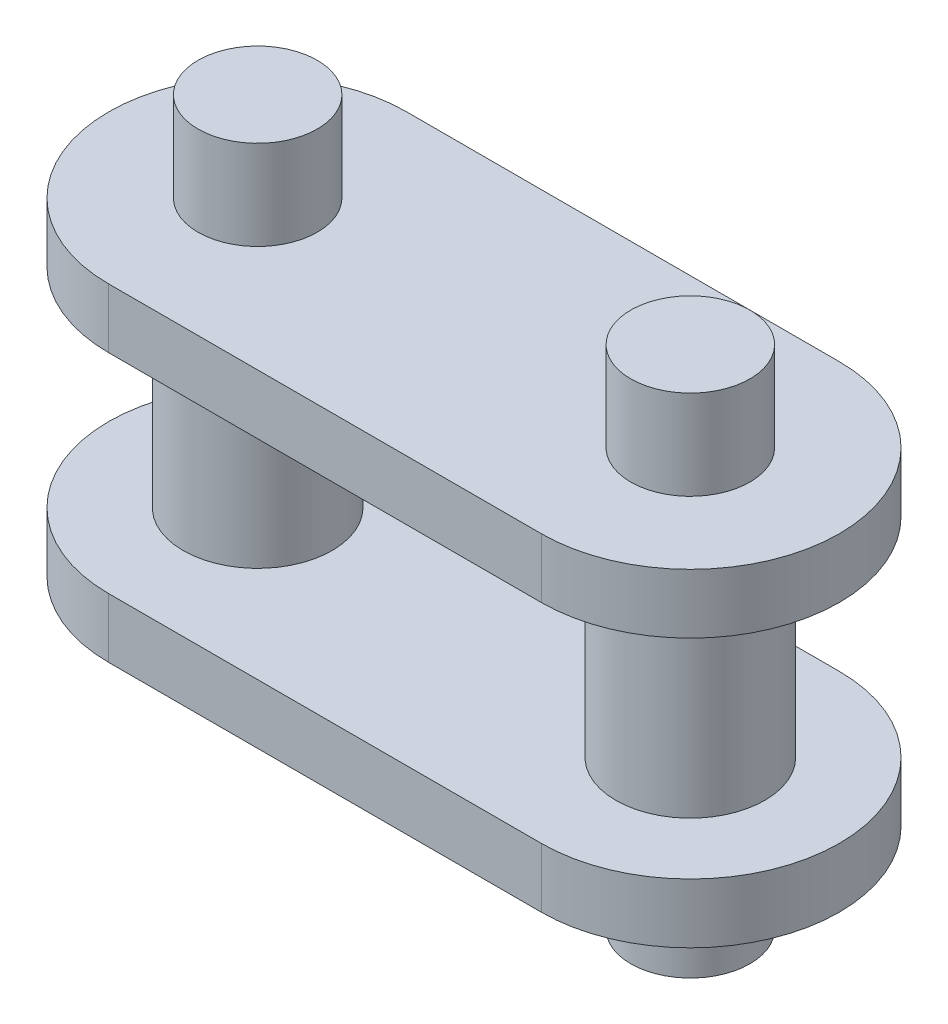
SolidWorks part; units mm, degrees
ref_plane "Front Plane" through (0, 0, 0) normal (0, 0, 1) x (1, 0, 0)
ref_plane "Top Plane" through (0, 0, 0) normal (0, 1, 0) x (1, 0, 0)
ref_plane "Right Plane" through (0, 0, 0) normal (1, 0, 0) x (0, 0, -1)
other "Configuration Table"
sketch "Sketch1" plane through (0, 0, 0) normal (0, 1, 0) x (1, 0, 0)
  line L0 (0, 0) -> (14.52, 0) construction
  line L1 (0, 5) -> (14.52, 5)
  line L2 (0, -5) -> (14.52, -5)
  arc A0 (0, 5) -> (0, -5) centre (0, 0) ccw
  arc A1 (14.52, -5) -> (14.52, 5) centre (14.52, 0) ccw
  point P3 (7.26, 0)
  dimension "D2" = 5
  dimension "D1" = 14.52
extrude "Boss-Extrude1" add sketch "Sketch1" along normal blind 2
sketch "Sketch2" plane through (0, 2, 0) normal (0, 1, 0) x (1, 0, 0)
  circle A0 centre (0, 0) radius 2.5
  circle A1 centre (14.52, 0) radius 2.5
  dimension "D1" = 5
  dimension "D2" = 5
extrude "Boss-Extrude2" add sketch "Sketch2" along normal blind 7
sketch "Sketch3" plane through (0, 9, 0) normal (0, 1, 0) x (1, 0, 0)
  line L0 (0, 0) -> (14.52, 0) construction
  line L1 (0, 5) -> (14.52, 5)
  line L2 (0, -5) -> (14.52, -5)
  arc A0 (0, 5) -> (0, -5) centre (0, 0) ccw
  arc A1 (14.52, -5) -> (14.52, 5) centre (14.52, 0) ccw
  point P4 (7.26, 0)
  dimension "D1" = 5
extrude "Boss-Extrude3" add sketch "Sketch3" along normal blind 2
sketch "Sketch4" plane through (0, 11, 0) normal (0, 1, 0) x (1, 0, 0)
  circle A0 centre (0, 0) radius 2
  circle A1 centre (14.52, 0) radius 2
  dimension "D1" = 4
  dimension "D2" = 4
extrude "Boss-Extrude4" add sketch "Sketch4" along normal blind 3
sketch "Sketch5" plane through (0, 0, 0) normal (0, -1, 0) x (1, 0, 0)
  circle A0 centre (0, 0) radius 2
  circle A1 centre (14.52, 0) radius 2
extrude "Boss-Extrude5" add sketch "Sketch5" along normal blind 3
ref_point "Point1"
ref_point "Point3"
ref_plane "Plane1" through (0, 5.5, 0) normal (0, 1, 0) x (1, 0, 0)
